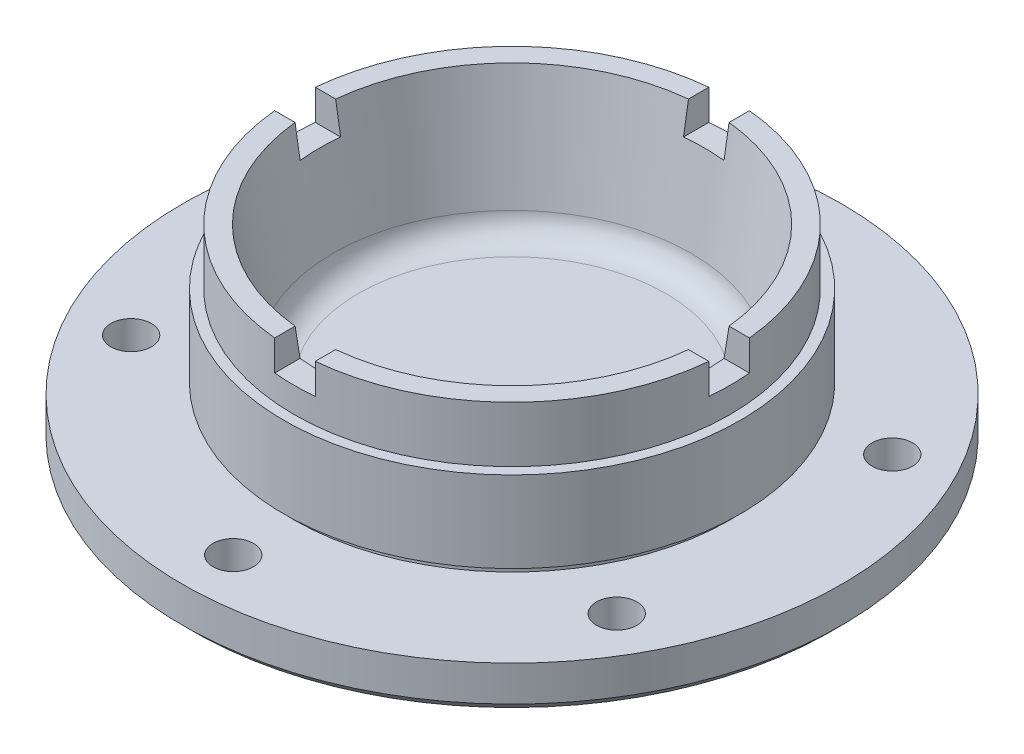
SolidWorks part; units mm, degrees
ref_plane "Front" through (0, 0, 0) normal (0, 0, 1) x (1, 0, 0)
ref_plane "Top" through (0, 0, 0) normal (0, 1, 0) x (1, 0, 0)
ref_plane "Right" through (0, 0, 0) normal (1, 0, 0) x (0, 0, -1)
sketch "Sketch2" plane through (0, 0, 0) normal (0, 0, 1) x (1, 0, 0)
  line L0 (65, 9) -> (65, 0)
  line L2 (0, 2) -> (29, 2)
  line L3 (29, 2) -> (31, 0)
  line L4 (65, 0) -> (31, 0)
  line L5 (65, 9) -> (43, 9)
  line L6 (43, 9) -> (43, 11)
  line L7 (43, 11) -> (45, 11)
  line L8 (45, 11) -> (45, 27)
  line L9 (45, 27) -> (43, 27)
  line L10 (43, 27) -> (43, 38)
  line L11 (43, 38) -> (39, 38)
  line L12 (35.3121, 15.4093) -> (39, 38)
  line L13 (0, 11) -> (30.3472, 11)
  line L14 (0, 2) -> (0, 11)
  arc A0 (35.3121, 15.4093) -> (30.3472, 11) centre (30.3472, 16) cw
  dimension "D14" = 5
  dimension "D1" = 65
  dimension "D3" = 29
  dimension "D5" = 22
  dimension "D6" = 9
  dimension "D7" = 2
  dimension "D8" = 2
  dimension "D9" = 16
  dimension "D10" = 2
  dimension "D11" = 11
revolve "Revolve1" add sketch "Sketch2" angle 360 about L14
sketch "Sketch3" plane through (0, 38, 0) normal (0, 1, 0) x (1, 0, 0)
  line L0 (55.9644, 4) -> (24.1821, 4)
  line L1 (-4, 55.9644) -> (4, 55.9644)
  line L2 (-4, 55.9644) -> (-4, 24.1821)
  line L3 (-4, 24.1821) -> (4, 24.1821)
  line L4 (4, 55.9644) -> (4, 24.1821)
  line L5 (55.9644, -4) -> (24.1821, -4)
  line L6 (55.9644, 4) -> (55.9644, -4)
  line L7 (24.1821, 4) -> (24.1821, -4)
  line L8 (4, -55.9644) -> (4, -24.1821)
  line L9 (-4, -55.9644) -> (-4, -24.1821)
  line L10 (4, -55.9644) -> (-4, -55.9644)
  line L11 (4, -24.1821) -> (-4, -24.1821)
  line L12 (-55.9644, -4) -> (-24.1821, -4)
  line L13 (-55.9644, 4) -> (-24.1821, 4)
  line L14 (-55.9644, -4) -> (-55.9644, 4)
  line L15 (-24.1821, -4) -> (-24.1821, 4)
  point P20 (0, 0)
  dimension "D1" = 8
  dimension "D2" = 4
  dimension "D3" = 4
extrude "Cut-Extrude1" cut sketch "Sketch3" against normal blind 6
chamfer "Chamfer1" distance 2 angle 45 1 edges at (0, 0, -65)
sketch "Sketch4" plane through (0, 38, 0) normal (0, 1, 0) x (1, 0, 0)
  line L0 (0, 0) -> (83.0953, 0) construction
  line L1 (0, 0) -> (0, 72.5426) construction
  line L2 (0, 0) -> (75.9687, 43.8606) construction
  line L3 (0, 0) -> (-76.86, 44.3751) construction
  circle A1 centre (0, 55) radius 4
  circle A2 centre (47.8177, 27.1748) radius 4
  circle A3 centre (-47.6314, 27.5) radius 4
  circle A4 centre (-47.6314, -27.5) radius 4
  circle A5 centre (0, -55) radius 4
  circle A6 centre (47.8177, -27.1748) radius 4
  dimension "D4" = 8
  dimension "D5" = 8
  dimension "D6" = 8
  dimension "D1" = 60
  dimension "D2" = 60
extrude "Cut-Extrude2" cut sketch "Sketch4" against normal blind 67
scale "Scale 1" bodies to scale 103 scale about centroid uniform scaling yes scale factor 1.875
